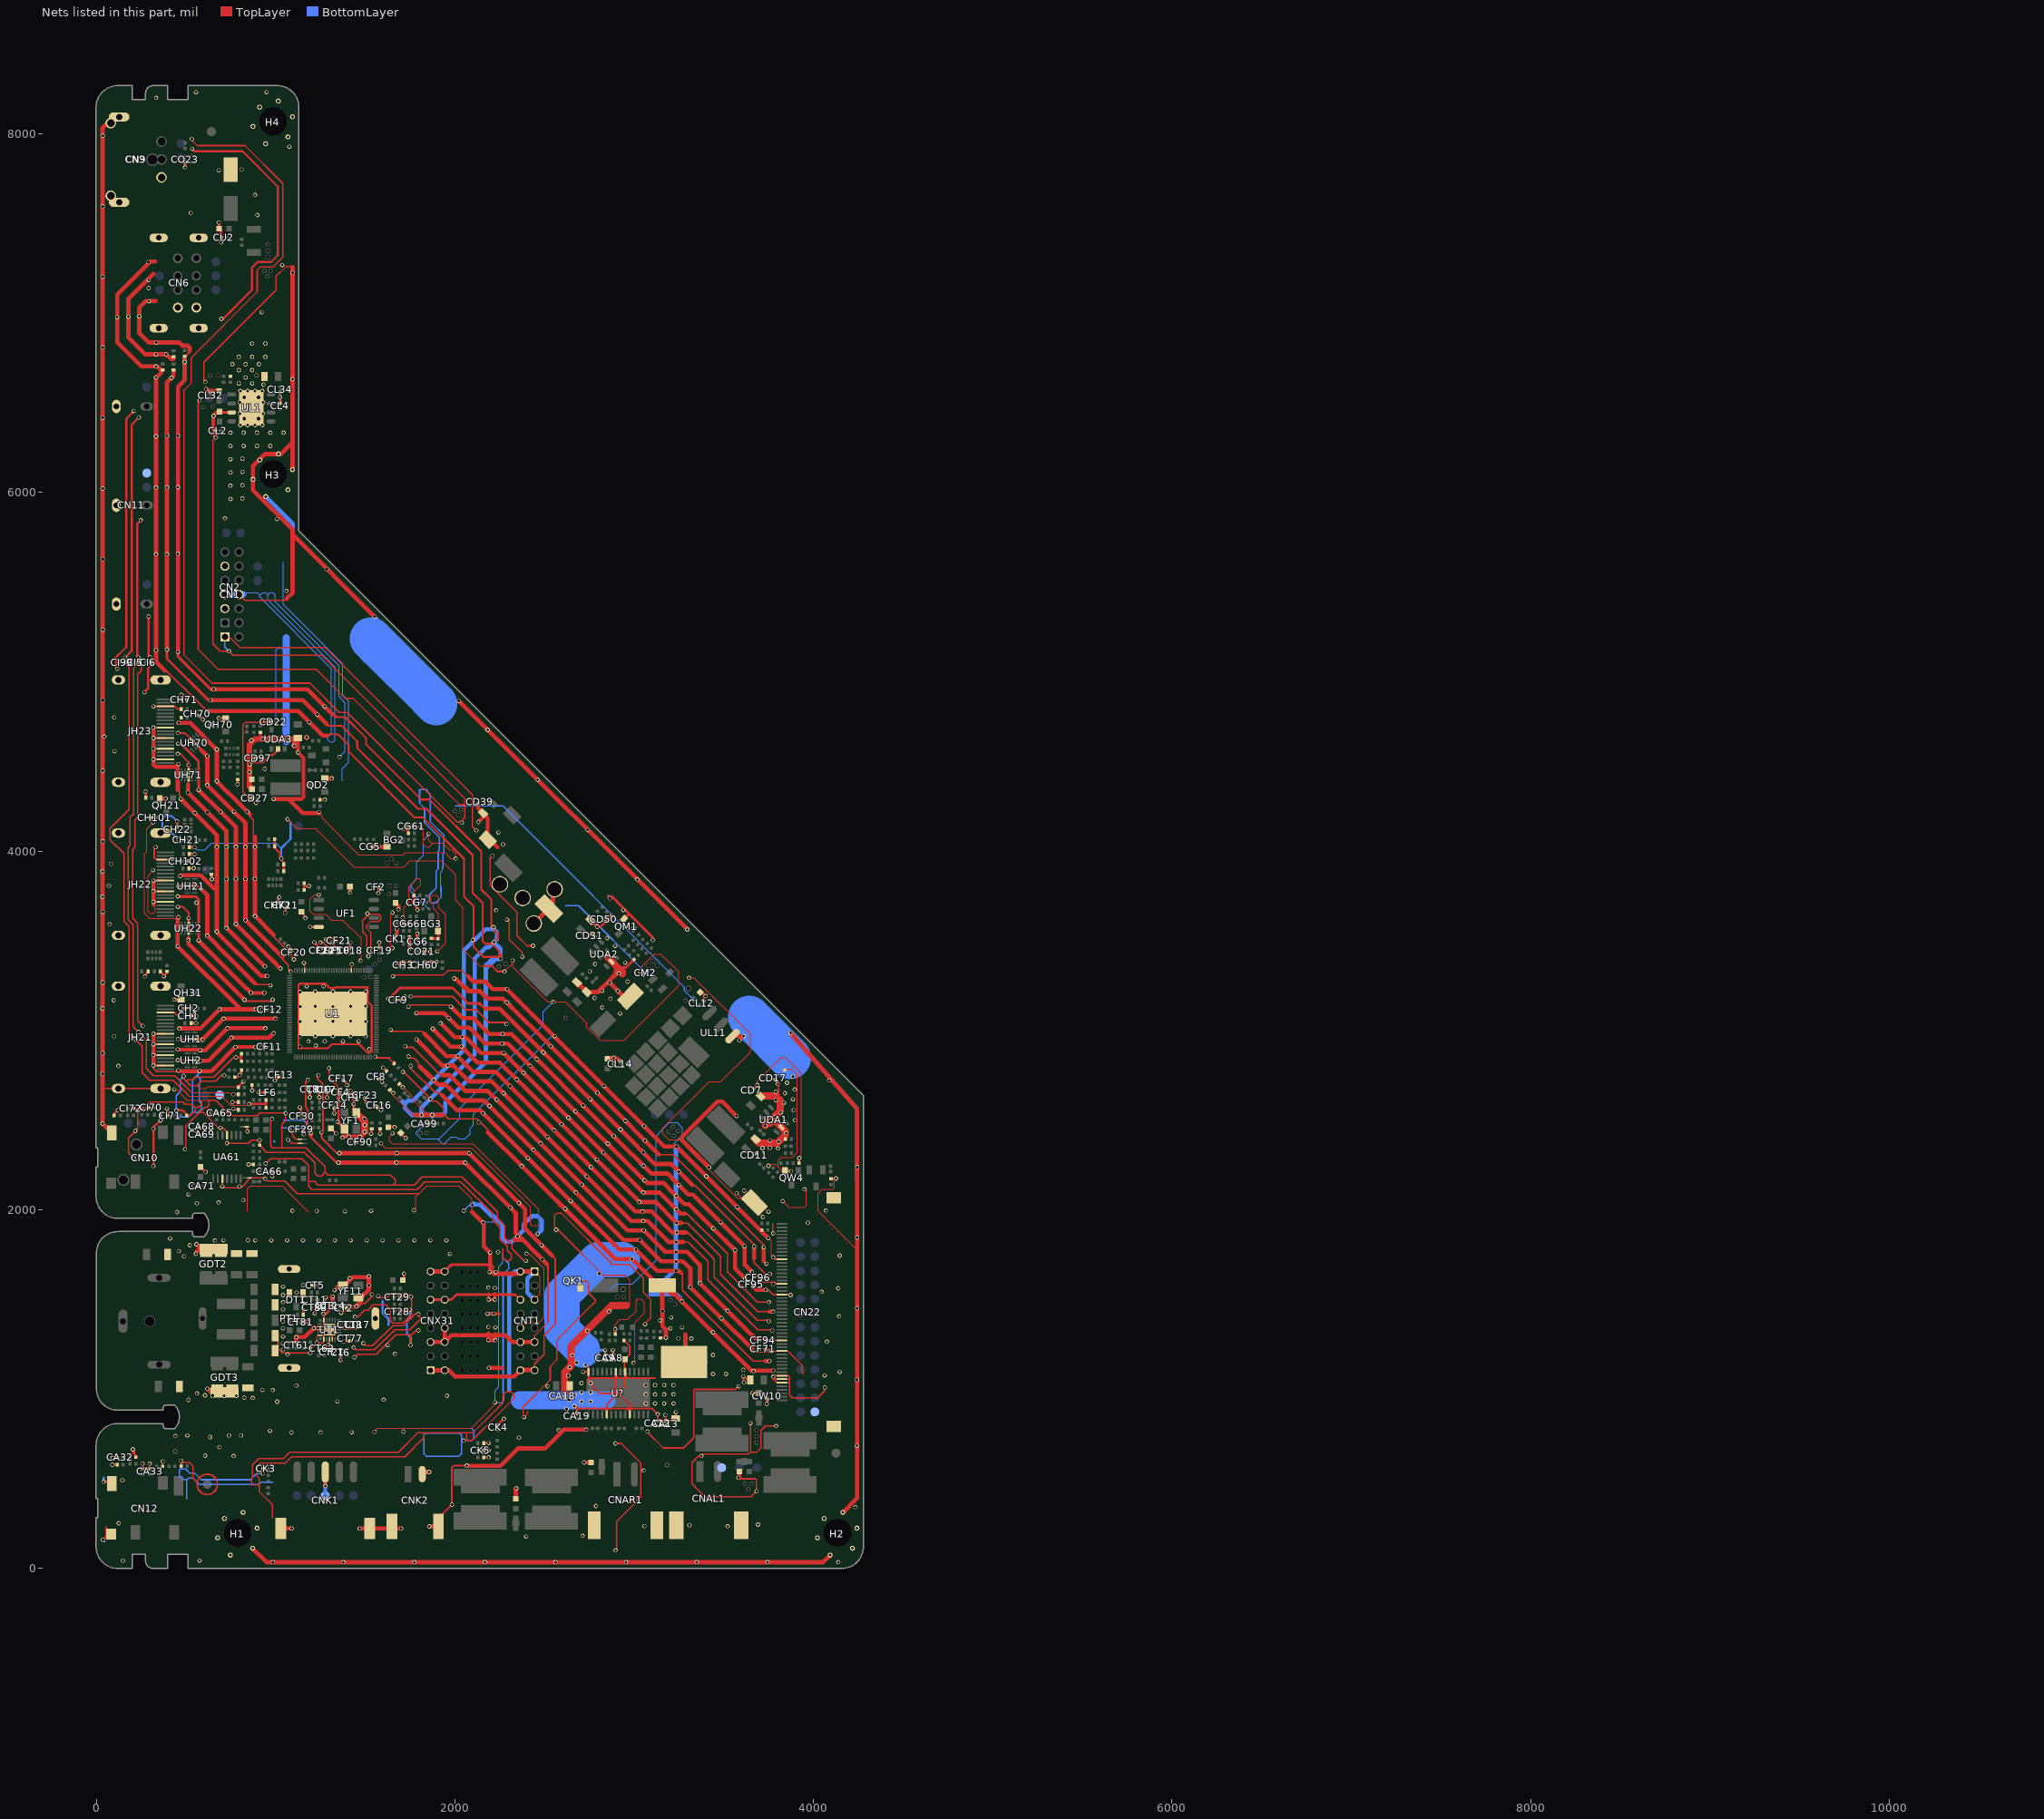
[diagram p0: the nets of this part, all layers, seen from the top]
# Altium PCB MISC105950.PcbDoc (part 7 of 15)
Units mil, origin at the board's own origin, x right, y up, seen from the top; angles counter-clockwise.
Board outline 4280.62 x 8272.76 mil, 2 copper layers (TopLayer, BottomLayer), stack 61.855 mil thick; 541 components, 268 nets, 2324 pads, 1157 vias.

## Via types
v1: diameter 23.62, hole 15.75, TopLayer to BottomLayer, tented both sides, 1087 vias
v2: diameter 23.62, hole 15.75, TopLayer to BottomLayer, 51 vias
v3: diameter 27.56, hole 19.68, TopLayer to BottomLayer, 15 vias
v4: diameter 31.5, hole 19.68, TopLayer to BottomLayer, tented both sides, 4 vias

## Nets (pads, with @x,y where several pads share a name; then routed paths per layer and width w, separated by ;. In a path a pad name is that pad's centre, name@x,y a point inside that pad or via, vN(x,y) a via of type N, cw(c..) or ccw(c..) an arc to the next point about the centre after c; other vN are vias at no path point) (continued)
GND: AV_GND.1 BG2.E BG3.E CA1.1 CA2.1 CA7.1 CA8.1 CA9.1 CA12.1 CA13.1 CA18.1 CA19.1 CA20.1 CA21.2 CA22.1 CA23.2 CA32.2@114.76,617 CA32.2@121.65,617 CA33.2@297,548.35 CA33.2@297,555.24 CA65.2@671.26,2539.5 CA65.2@678.15,2539.5 CA66.1 CA68.2@568.93,2461.69 CA68.2@575.82,2461.69 CA69.2@568.93,2420 CA69.2@575.82,2420 CA70.2 CA71.2@568.61,2131.5 CA71.2@575.5,2131.5 CA99.1 CD7.2@3661.5,2671 CD7.2@3666.37,2675.87 CD11.1 CD17.2@3780.46,2727.54 CD17.2@3785.33,2722.67 CD22.1 CD25.1 CD26.1 CD27.1 CD30.1 CD31.2@2755.96,3534.46 CD31.2@2760.83,3539.33 CD39.2@2126.67,4262.67 CD39.2@2131.54,4267.54 CD50.2@2835.96,3612.04 CD50.2@2840.83,3607.17 CD53.2 CD54.2 CD57.2 CD77.1 CD96.1 CD97.2@884.04,4517.5 CD97.2@890.93,4517.5 CD99.2 CD101.A CD102.A CF1.1 CF2.1 CF3.1 CF4.1 CF5.1 CF6.1 CF7.1 CF8.1 CF9.1 CF10.1 CF11.2@946.54,2907 CF11.2@953.43,2907 CF12.1 CF13.1 CF14.1 CF15.1 CF16.1 CF17.1 CF18.2@1414,3454.35 CF18.2@1414,3461.24 CF19.2@1577,3455.84 CF19.2@1577,3462.73 CF20.1 CF21.2@1335.43,3500.5 CF21.2@1342.32,3500.5 CF23.1 CF24.1 CF25.2@1299.5,3454.18 CF25.2@1299.5,3461.07 CF29.2@1149.35,2447 CF29.2@1156.24,2447 CF30.2@1144.5,2530.07 CF30.2@1144.5,2536.96 CF58.1 CF59.1 CF71.1 CF90.2@1452.26,2377 CF90.2@1459.15,2377 CF94.1 CF95.1 CF96.1 CG5.1 CG6.1 CG7.1 CG61.1 CG66.1 CH1.2@522.35,3081 CH1.2@529.24,3081 CH2.2@495.76,3123 CH2.2@502.65,3123 CH3.1 CH21.2@483.61,4062.1 CH21.2@490.5,4062.1 CH22.2@449.5,4131.35 CH22.2@449.5,4138.24 CH60.1 CH70.2@568.47,4758.03 CH70.2@573.35,4753.15 CH71.2@498.34,4843.5 CH71.2@505.23,4843.5 CH72.1 CH101.1 CH102.1 CI5.1 CI6.1 CI70.1 CI71.1 CI72.1 CI99.1 CK1.1 CK3.2@928.26,554.5 CK3.2@935.15,554.5 CK4.1 CK5.1 CK11.2@1053.5,3681.67 CK11.2@1053.5,3688.56 CL1.1 CL2.1 CL4.2@1023.5,6492.85 CL4.2@1023.5,6499.74 CL10.2 CL11.1 CL12.1 CL13.1 CL14.1 CL31.2 CL32.2@635.43,6553.11 CL32.2@635.43,6560 CL34.1 CM2.1 CN1.1 CN1.5 CN1.7 CN1.8 CN1.11 CN2.3 CN2.5 CN2.6 CN2.9 CN3.2 CN3.3 CN6.4 CN6.8 CN6.9 CN6.10 CN6.11 CN6.12 CN9.3 CN9.4 CN9.5 CN10.2 CN11.2 CN11.4 CN11.6 CN12.1 CN12.2 CN22.6 CN22.7 CN22.8 CN22.15 CN22.18 CN22.31 CN22.34 CN22.41 CN22.52 CN22.53 CNAL1.3 CNAL1.4 CNAR1.3 CNAR1.4 CNK1.3 CNK1.6 CNK1.7 CNK2.2 CNK2.3 CNK2.4 CNT1.1 CNT1.2 CNT1.5 CNT1.6 CNT1.10 CNT1.11 CNT1.12 CNT1.15 CNT1.16 CNX31.1 CNX31.2 CNX31.5 CNX31.6 CNX31.8 CNX31.11 CNX31.12 CNX31.15 CNX31.16 CO21.1 CO23.1 CT2.1 CT3.1 CT5.2@1200.76,1577 CT5.2@1207.65,1577 CT6.1 CT8.1 CT10.2@1241,2652.76 CT10.2@1241,2659.65 CT11.1 CT14.1 CT17.2@1455,1340.76 CT17.2@1455,1347.65 CT18.1 CT21.1 CT28.1 CT29.2@1686.85,1510.5 CT29.2@1693.74,1510.5 CT41.1 CT42.1 CT43.1 CT44.1 CT45.2 CT46.2 CT47.2 CT48.2 CT49.2 CT50.2 CT51.2 CT52.2 CT53.2 CT61.2@1114.5,1252.35 CT61.2@1114.5,1259.24 CT62.2@1266.35,1224.5 CT62.2@1273.24,1224.5 CT77.1 CT80.1 CT81.2@1146.85,1372.5 CT81.2@1153.74,1372.5 CT88.2@1224.83,1453.9 CT88.2@1231.72,1453.9 CU1.1 CU2.2@694.26,7423.88 CU2.2@701.15,7423.88 CW9.1 CW10.1 DA51.A DA52.A DA53.A DH1.A DH2.A DH3.A DH4.A DH21.A DH22.A DH23.A DH70.A DH71.A DH72.A DH73.A DH74.A DH75.A DH76.A DH81.A DI2.A DI3.A DI22.A DI23.A DI24.A DI33.A DI34.A DK2.A DK3.A DK4.A DK70.A DM4.A DO21.A DT1.1 DT1.3 DU1.A DU2.A DU11.A DU12.A DU31.A DU32.A DU33.A DU34.A EA1.2 EA33.2 EA34.2 ED6.2 EU1.2 GDT2.2@613,1754.07 GDT2.2@653,1779.67 GDT2.2@693,1754.07 GDT3.2@674.5,1004.93 GDT3.2@714.5,979.33 GDT3.2@754.5,1004.93 GND_AMP.1 GND_KEY.1 GND_TP.1 H1.1 H1.2 H1.3 H1.4 H1.5 H1.6 H2.1 H2.2 H2.3 H2.4 H2.5 H2.6 H3.1 H3.2 H3.3 H3.4 H3.5 H3.6 H4.1 H4.2 H4.3 H4.4 H4.5 H4.6 HSA1.1 JH21.2 JH21.5 JH21.8 JH21.11 JH21.17 JH21.20 JH21.21 JH21.22 JH21.23 JH22.5 JH22.8 JH22.11 JH22.17 JH22.20 JH22.21 JH22.22 JH22.23 JH23.2 JH23.5 JH23.8 JH23.11 JH23.17 JH23.20 JH23.21 JH23.22 JH23.23 LF6.1 LT2.1 LT4.1 pad.VIA5@747,5964 pad.VIA5@747,6038 pad.VIA5@747,6112 pad.VIA5@747,6186 pad.VIA5@747,6260 pad.VIA5@747,6334 pad.VIA5@757.5,6716 pad.VIA5@793.5,6609 pad.VIA5@793.5,6683 pad.VIA5@793.5,6757 pad.VIA5@813.5,5967 pad.VIA5@813.5,6041 pad.VIA5@813.5,6115 pad.VIA5@813.5,6189 pad.VIA5@821,6260 pad.VIA5@821,6334 pad.VIA5@831.5,6642 pad.VIA5@831.5,6716 pad.VIA5@867.5,6609 pad.VIA5@867.5,6683 pad.VIA5@867.5,6757 pad.VIA5@867.5,6831 pad.VIA5@895,6260 pad.VIA5@895,6334 pad.VIA5@905.5,6716 pad.VIA5@941.5,6757 pad.VIA5@941.5,6831 pad.VIA5@969,6260 pad.VIA5@969,6334 pad.VIA5@1043,6334 pad.VIA5@2250,3814.5 pad.VIA5@2377,3738 pad.VIA5@2439.5,3595.5 pad.VIA5@2555.5,3786.5 pad.VIA5@2622.57,886.29 pad.VIA5@2632.07,1073.5 pad.VIA5@2639.5,1120 pad.VIA5@2654,1186.93 pad.VIA5@2665.57,966.5 pad.VIA5@2665.86,903 pad.VIA5@2679,1145.43 pad.VIA5@2704.98,928.64 pad.VIA5@2704.98,980.07 pad.VIA5@2704.98,1031.51 pad.VIA5@2737.5,1322.93 pad.VIA5@2756.41,928.64 pad.VIA5@2756.41,980.07 pad.VIA5@2756.41,1031.51 pad.VIA5@2860.15,1431.85 pad.VIA5@3064,917.67 pad.VIA5@3064,969.1 pad.VIA5@3064,1020.53 pad.VIA5@3115.43,917.67 pad.VIA5@3115.43,969.1 pad.VIA5@3115.43,1020.53 pad.VIA5@3166.87,917.67 pad.VIA5@3166.87,969.1 pad.VIA5@3166.87,1020.53 pad.VIA5@3201,1337 pad.VIA5@3218.3,917.67 pad.VIA5@3218.3,969.1 pad.VIA5@3218.3,1020.53 pad.VIA5@3318,1280 pad.VIA5@3439,1188.5 pad.VIA5@3439.21,1082.36 pad.VIA5@3511,1082 PT1.2 PT1.3 PT1.4 QD2.E QH21.E QH31.E QH70.E QK1.E QM1.E QW4.E RA1.2 RA4.JP_2K RA5.JP_2K RA9.1 RA11.1 RA55.1 RA56.1 RA64.JP_2K RA65.JP_2K RA69.1 RA71.1 RD28.1 RD35.1 RD47.2 RD53.2 RD54.1 RD88.1 RF5.1 RF12.2 RF13.2 RF19.2 RG8.1 RG9.1 RH2.2 RH75.2 RH82.2 RI14.2 RI16.2 RI21.1 RI23.1 RI25.1 RI36.1 RL32.1 RO22.1 RW11.1 RW14.2 U1.105 U1.124 U1.EPAD U?.6 U?.8 U?.14 U?.19 U?.24 UA61.4 UA61.10 UDA1.2 UDA2.2 UDA3.2 UF1.4 UH1.GND UH2.GND UH21.GND UH22.GND UH70.GND UH71.GND UL1.3 UL1.EPAD UL11.1 UT1.2 UT1.4 UT1.5 UT1.11 UT1.18 UT1.21 UT1.22 UT1.24 UT1.EPAD YF1.2 YF1.4 YF11.2 YF11.4 YPbPr_GND.1 | length 228401.4
  TopLayer w5: 302.82,3624.68 295.33,3624.68 266.69,3653.32 266.69,3982.99 279.5,3995.8 279.5,4124.14 314.86,4159.5 v1(315.5,4159.5) ; 479.91,6818.97 489.41,6809.47 504.93,6809.47 ; DU1.A@491,6759.65 DU1.A@491,6762.82 ; 501.41,2613 504.72,2609.69 659.31,2609.69 ; 511.56,2637.5 511.56,2636.09 515.96,2631.69 696.81,2631.69 747.83,2580.67 842.99,2580.67 v1(851.16,2588.84) ; DH70.A@515.23,3903.1 540.98,3903.1 v1(541.9,3904.02) ; CH102.1@517.07,3943.6 543.63,3943.6 v1@543.73,3943.5 ; 520.44,2662.56 529.31,2653.69 741.31,2653.69 v1@755,2640 ; 560.6,2691.37 576.28,2675.69 607.69,2675.69 618,2686 786.77,2686 RI21.1@790.27,2682.5 ; 842.38,1988.45 842.38,2118.37 855.86,2131.85 1023.65,2131.85 1036.33,2131.85 1181.38,1986.79 ; 864.5,2589 882,2589 ; v1@1240.5,4211.5 1258.52,4193.48 1258.52,4182.98 1462,3979.5 1709.14,3979.5 1719.95,3990.31 ; v1(1550,759.5) 1570.35,779.85 2090.96,779.85 2145.06,833.94 ; DU33.A@1636.33,2668.17 1654,2650.5 1654,2637.4 1770.2,2521.2 ; v1@1641.84,3457 1641.84,3524.5 ; 1641.84,3630.84 1641.84,3604 ; v1(1651.16,3458.36) 1641.84,3467.67 1641.84,3524.5 ; v1(1651.16,3656.01) 1651.16,3654.16 1641.84,3644.84 1641.84,3604 ; CF15.1@1674,3701.5 CF15.1@1674,3718.5 ; v1@1678,3371 1686,3371 1695.23,3380.23 CH3.1@1709.5,3380.23 ; 1706.95,3977.31 1719.95,3990.31 ; CH3.1@1710.5,3381.23 RH82.2@1749.5,3381.23 RH82.2@1749.5,3385.26 ; CG66.1@1712.27,3595 1712.27,3625.23 1715.68,3628.63 1715.68,3684.18 1742.91,3711.41 1742.91,3802.1 1769.6,3828.79 1769.6,3832.6 1783,3846 1798.5,3846 1809.5,3835 1809.5,3812.69 ; v1@1713.03,2680.03 1760.93,2632.13 1760.93,2624.82 1759.83,2623.72 1759.83,2617.83 1846,2531.66 ; v1(1745,3452.5) v1@1745.23,3452.73 ; 1780,1986.79 1780,2071.74 1840.11,2131.85 2020.58,2131.85 2094.93,2057.5 v1(2094.93,2025) 2094.93,1986.79 ; v1@1792,3676.5 1769.77,3698.73 RG9.1@1769.77,3752 1769.77,3772.96 1809.5,3812.69 ; 1797.15,3800.35 1809.5,3812.69 ; v1(1808,4136) 1822.69,4121.31 1822.69,4036.5 1838.69,4020.5 1855,4020.5 1880,4045.5 ; CH60.1@1828.5,3374.34 RH2.2@1861.61,3374.34 ; v1(1852,4095.5) 1852,4061.81 1868.31,4045.5 1880,4045.5 ; RH2.2@1868.5,3381.23 1896.27,3381.23 v1(1896.5,3381) ; 2152.56,841.44 2145.06,833.94 ; v1(2222.61,924.66) 2226.82,920.44 2231.56,920.44 2145.06,833.94 ; v1(2275,3328) 2321.5,3374.5 v1(2321.5,3389) 2321.5,3353.5 2517,3158 v1(2548,3158) ; 2607.59,3158 v1(2548,3158) ; HSA1.1@3193.65,1175.35 3355.65,1175.35 HSA1.1@3383,1148 ; 3249,3324.61 3249,3250 2941.38,2942.39 2810.11,2942.39 2734.39,3018.11 2734.39,3040.42 2616.81,3158 v1(2548,3158) ; 3653.11,1214.27 3663.24,1204.14 3761.94,1204.14 v1@3768.62,1210.82 ; v1(3746.74,1840.63) 3765.5,1821.87 3765.5,1743.65 v1@3775.92,1733.23 ; 1641.84,3524.5 1641.84,3604 ; 1719.95,3990.31 1944.19,3990.31 1976.5,3958 v1(2004,3958) 2004,3985.81 1984,4005.81 1970.19,4005.81 1930.5,4045.5 1880,4045.5
  TopLayer w6: 302.82,3624.68 v1@448.84,3624.68 ; v1(314.5,3893.5) 314.5,3890.35 287.19,3863.04 287.19,3661.81 297,3652 315.02,3652 ; 315.21,3652.19 326.81,3663.79 326.81,3671.81 326.94,3671.94 326.94,3706.8 ; 1078.88,4163.62 v1(1065,4177.5) 1116.5,4126 1222,4126 1436.5,3911.5 1625.5,3911.5 ; 1191.97,3731.62 1191.97,3718 ; 1229,1281.53 1229,1293 1234.5,1298.5 UT1.EPAD@1268,1298.5 ; v1(1240.5,3756.5) 1215,3756.5 1191.97,3733.47 1191.97,3718 ; v1@1470.98,3387.23 1470.98,3400.76 1475.81,3405.6 1475.81,3512.77 1373.15,3615.43 1309.94,3615.43 1279.06,3646.31 1209.81,3646.31 1191.97,3664.15 1191.97,3718 ; v1@1585.63,2364.63 v1@1585.63,2374.19 ; v1(1586,2369) 1610.5,2344.5 2091.48,2344.5 2421,2014.98 2421,1918.31 2427,1912.31 2465.31,1912.31 2465.5,1912.5 ; 1637.5,3911.5 1625.5,3911.5 ; v1(1650.76,2425.26) 1633.81,2408.32 1633.81,2380.69 1649,2365.5 2100.17,2365.5 2465.5,2000.17 2465.5,1892.5 ; DO21.A@1867.5,3512.23 1904,3512.23 v1@1904,3594.5 ; v1@1900.5,3440.5 1946.5,3486.5 1946.5,3644.97 1906,3685.47 1906,3740.5 1894.19,3752.31 1870.31,3752.31 1863.5,3745.5 1863.5,3715 1878,3700.5 1878,3679 1907,3650 1907,3514.23 RO22.1@1904.5,3511.73 ; 2188,3358.5 2137,3358.5 2043.81,3451.69 2043.81,3683.6 2002,3725.41 2002,3867.97 1925.16,3944.81 1747.31,3944.81 1714,3911.5 1625.5,3911.5 ; CNT1.10@2364.47,1339.15 2394.12,1368.8 2467.8,1368.8 2496,1397 2496,1670.08 2412.58,1753.5 v1(2398,1753.5) ; CNT1.2@2364.47,1654.11 CNT1.1@2443.21,1654.11 2475,1622.32 2475,1528.42 CNT1.5@2443.21,1496.63 ; CNT1.11@2443.21,1260.41 2443.21,1297.21 2519,1373 2519,1374.42 ; v1(2460,1863.5) 2465.5,1869 2465.5,1892.5 ; 2465.5,1884.38 2465.5,1892.5 ; v1@2893.67,1333.33 2893.67,1359.67 2920,1386 2963.26,1386 3009.5,1432.24 3009.5,1492 3018.5,1501 3037.33,1501 ; 2950.08,1632 2974.5,1607.58 2974.5,1466.5 ; v1(2995.99,1143.72) 3003.63,1151.36 3003.63,1319.5 ; 3003.63,1348.42 3003.63,1319.5 ; 3010,1489.5 3021.5,1501 3037.33,1501 ; v1(3031,3329) 3043.59,3341.59 3043.59,3356.41 3112.69,3425.5 3148.11,3425.5 3249,3324.61 ; CM2.1@3051.67,3310.17 CM2.1@3051.67,3315.83 ; v1(3054.46,2465.14) 3064.55,2455.05 3069.55,2455.05 ; v1@3059.83,2464.77 3069.55,2455.05 ; 3164.1,2360.5 3069.55,2455.05 ; 3276.46,2375.96 3263.93,2388.5 ; 3287.1,2352.6 3575.7,2064 ED6.2@3646,2064 ; v1(3305.5,3292.5) 3316.5,3292.5 3317,3293 3332,3293 3647,2978 3647,2878.56 3481.44,2713 3417.87,2713 3158.08,2453.21 3158.08,2423.74 3193.32,2388.5 3237.62,2388.5 ; v1(3572,2091) 3623.56,2039.44 ED6.2@3670.56,2039.44 ; v1(3613,2105) 3670.56,2047.44 ED6.2@3670.56,2039.44 ; CD99.2@3677.11,2392.67 3677.11,2377.39 3698,2356.5 ; v1@3690.53,2700.03 v1(3685.5,2695) 3685.5,2715.95 3816.55,2847 3843.53,2847 3931.1,2759.43 3931.1,2313.5 ; v1(3717,1958) 3670.56,2004.44 ED6.2@3670.56,2039.44 ; v1(3748,1987.5) 3696.06,2039.44 ED6.2@3670.56,2039.44 ; v1(3748,2244) 3756.56,2252.56 3785.44,2252.56 3801.68,2236.32 ; 3777.5,2493.46 UDA1.2@3804.98,2465.98 ; v1(3827.64,2046.86) 3863,2011.5 3948,2011.5 3958.5,2022 3958.5,2072.5 ; 3835.86,2435.1 UDA1.2@3804.98,2465.98 ; RD28.1@3838.98,2778.52 3844.98,2784.52 3876.32,2784.52 3910.1,2750.73 3910.1,2319.06 3882.04,2291 3819.52,2291 3801.68,2273.15 3801.68,2236.32 ; QW4.E@3840.5,2216 3822,2216 3801.68,2236.32 ; 3853.5,2390.5 3853.5,2417.46 UDA1.2@3804.98,2465.98 ; v1@3919.5,2286 3931.1,2297.6 3931.1,2313.5 ; 3931.1,2297.5 3931.1,2313.5 ; v1(3949,2113) 3958.5,2103.5 3958.5,2072.5 ; 3958.5,2081.5 3958.5,2072.5 ; 4112.77,2121.27 4106.14,2114.64 ; 4115.34,2127.07 4115.34,2154.01 ; v1(4125.15,2172.73) RW11.1@4097.5,2172.73 4097.5,2171.86 4115.34,2154.01 ; 4243.09,1784 4232.17,1784 4024.5,1991.67 4024.5,2091 4048.14,2114.64 4106.14,2114.64 ; 3003.63,1319.5 3003.63,1370.68 3055.45,1422.5 3055.45,1482.87 3037.33,1501 ; 3237.62,2388.5 3263.93,2388.5 ; 3237.62,2388.5 3242.03,2392.91 3245.34,2392.91 3247.23,2391.02 3266.45,2391.02 3263.93,2388.5 ; 4106.14,2114.64 4115.34,2123.84 4115.34,2154.01
  TopLayer w7: CI99.1@155.01,5050.33 181.31,5024.03 181.31,5008.84 ; 179.47,4229 75.5,4125.03 75.5,4063.5 152.5,3986.5 152.5,3605.87 180.5,3577.87 180.5,2985.5 v1(219,2947) 254,2912 254,2764.5 297.21,2721.29 427.77,2721.29 511.56,2637.5 ; 181.31,4229 181.31,5008.84 ; 181.31,5011.69 181.31,5008.84 ; 205.31,4206.5 187,4188.19 187,4029.03 176.5,4018.53 176.5,3615.81 204.5,3587.81 204.5,3020 278,2946.5 278,2785.5 318.21,2745.29 437.71,2745.29 520.44,2662.56 ; 205.31,4207 205.31,5021.03 233.73,5049.45 CI5.1@233.73,5052 250.5,5035.23 250.5,5006 229.31,4984.81 229.31,4189.81 214,4174.5 214,4020.81 200.5,4007.31 200.5,3625.75 228.5,3597.75 228.5,3053.5 v1(257.5,3024.5) ; CI72.1@207.23,2564 229,2564 ; v1(207.5,2286.5) 177.5,2316.5 177.5,2400 v1(216,2438.5) 229,2451.5 229,2564 ; CI70.1@283.77,2564 229,2564 ; CI70.1@288.27,2568.5 288.27,2591.27 295.5,2598.5 481.22,2598.5 493.03,2586.69 532.59,2586.69 550.09,2569.19 ; v1(317,2803) 317,2787.27 334.42,2769.85 v1@448.34,2769.85 ; v2@446.67,1983.5 v2(448.81,1985.65) ; 461.61,4383.82 461.61,4311.02 510.05,4262.58 510.05,4250.55 ; v1@486,2743 486,2730.94 525.57,2691.37 560.6,2691.37 584.6,2715.37 664.09,2715.37 697.72,2749 v1(711.6,2749) ; v1(492.75,2336.25) 498,2341.5 498,2465.53 602.16,2569.69 613.91,2569.69 625.81,2581.59 625.81,2608.5 626,2608.69 ; 501.97,2714.97 509.69,2722.69 534.41,2722.69 551.1,2739.37 654.15,2739.37 ; DI24.A@502.46,2524.5 523.03,2524.5 550.09,2551.56 550.09,2569.19 ; 585,2608.69 585,2587.28 566.91,2569.19 550.09,2569.19 ; 611.5,2739.37 654.15,2739.37 ; 617,2608.69 663.99,2608.69 748.68,2524 781.5,2524 ; v1(691,2456) v1@693.5,2453.5 ; v1(701.5,2129.5) 701.59,2129.59 UA61.10@701.59,2171.5 701.59,2133.87 715.5,2119.96 804.37,2119.96 815.46,2131.04 ; 723.5,2549.18 723.5,2541.36 740.86,2524 781.5,2524 ; v1(727.18,2370.82) 729,2369 846,2369 864,2387 v1(909,2387) ; v1(763,2642.5) DI22.A@789.77,2642.5 ; v1(778.54,2848.54) 763.31,2848.54 654.15,2739.37 ; v1(797.5,2128.5) 812.91,2128.5 815.46,2131.04 ; 854.96,4205.46 854.96,4193.44 875,4173.4 875,4101.5 ; RA65.JP_2K@857.75,2173.34 815.46,2131.04 ; RA65.JP_2K@860.41,2176 932,2176 v1@941,2167 ; v1(868.16,2664.16) v1@870.5,2666.5 ; 875,4050 875,4101.5 ; 875,4085 875,4101.5 ; 876.73,3268.5 891.41,3253.81 966.85,3253.81 v1(970.35,3250.31) ; RA69.1@909.23,2359.25 949.14,2319.34 1158.78,2319.34 1218.11,2260.02 1218.11,2203.12 1233.72,2187.5 1253.5,2187.5 1274.5,2208.5 ; v1(941,2171) 952.15,2159.85 1047.92,2159.85 1071.58,2136.19 ; v1(943,2256.5) 970.84,2284.34 1144.29,2284.34 1183.11,2245.52 1183.11,2130.89 1201.81,2112.19 1787.93,2112.19 1830.58,2154.85 2031.52,2154.85 2209.84,1976.53 2209.84,1941.31 2251.69,1899.46 2251.69,1833.46 2291.19,1793.96 2291.19,1772.23 2314.5,1748.92 2314.5,1725.28 2302.41,1713.19 2285.59,1713.19 2266.19,1732.59 2266.19,1781 ; 962.24,3545.74 1086.21,3421.76 1086.21,3409.47 v1@1102.38,3393.3 ; 978.34,3403.77 1032.5,3349.61 1027.26,3344.37 v1(1025.69,3344.37) ; v1(978.5,2505) 972.5,2505 969.5,2502 969.5,2356.84 982,2344.34 1169.14,2344.34 ; 1035,2344.34 1035,2475.47 1054.66,2495.13 v1(1054.66,2537.66) 910.25,2537.66 896.59,2524 781.5,2524 ; 1036.74,3408.3 1036.74,3396.28 1070,3363.02 1070,3340.38 v1(1082.78,3327.6) ; 1059.08,2148.7 1071.58,2136.19 ; v1@1076.5,2389.5 v1(1068,2389.5) 1089.16,2368.34 RA4.JP_2K@1136.8,2368.34 ; v1(1092.5,2450) 1095,2447.5 1095,2408.78 1111.43,2392.34 RA5.JP_2K@1134.8,2392.34 RA5.JP_2K@1133.66,2392.34 ; 1118.74,2344.34 1169.14,2344.34 ; 1187.42,2155.81 1215.91,2155.81 1234.53,2137.19 1772.18,2137.19 1816.99,2182 2039.72,2182 2215.31,2006.41 ; v1(1216.5,1420.5) v1@1218,1422 ; v1@1220.42,1330 UT1.22@1246.35,1330 UT1.EPAD@1299.5,1330 ; v1@1221.1,1345.75 UT1.21@1246.35,1345.75 UT1.EPAD@1283.75,1345.75 ; RD47.2@1247.23,4287 v1(1274,4287) ; 1260.78,1256.5 1268,1263.72 UT1.2@1268,1276.85 1268,1298.5 UT1.EPAD@1299.5,1330 ; v1(1265.5,1419.5) 1265.62,1419.62 1283.38,1419.62 ; CT3.1@1278.5,1484.91 v1(1278.5,1509) ; UT1.EPAD@1280.8,1345.75 1268.63,1357.92 1268.63,1382.52 UT1.18@1268,1383.15 1268,1404.24 1283.38,1419.62 ; 1294.34,1469.07 1294.34,1430.58 1283.38,1419.62 ; v2@1295.48,1246 v2(1294.25,1244.78) 1299.5,1250.02 UT1.4@1299.5,1276.85 ; v1(1296.85,2788.14) 1296.85,2737.07 1342.81,2691.11 1342.81,2614.19 1347.5,2609.5 ; UT1.5@1315.25,1277.85 UT1.EPAD@1315.25,1315.25 ; v1@1315.5,1504.97 1315.5,1499 1317.5,1497 CT14.1@1317.5,1472.23 ; v1@1347.5,2486 1347.5,2522.5 ; v1@1347.5,2487.27 YF1.4@1382.57,2452.2 ; v1@1360,1422.11 1370.39,1432.5 1380.5,1432.5 ; v1(1361,1160) 1361,1186.27 CT6.1@1361.5,1186.77 ; v1(1364.5,1423) 1371,1423 1380.5,1432.5 ; YF1.4@1382.57,2471.89 YF1.4@1382.57,2476.93 ; v1(1384.5,1338.5) v1@1386.77,1340.77 ; v1@1387,1337 1381.5,1337 1372.75,1345.75 UT1.11@1352.65,1345.75 1315.25,1345.75 UT1.EPAD@1299.5,1330 ; CT2.1@1393.23,1450 1406.23,1463 1441.5,1463 YF11.4@1470.31,1491.81 ; v1@1444,1408 1442,1406 v1(1442,1402) 1458.24,1402 1493.85,1437.61 1513.67,1437.61 1543.56,1467.5 1563,1467.5 ; 1446,1218.5 v1(1434.5,1230) 1448,1216.5 1550.97,1216.5 1662.97,1328.5 1747.47,1328.5 1805.97,1387 1805.97,1398.53 v1@1787.53,1416.97 ; CT17.2@1451.24,1337 CT17.2@1455,1340.76 ; 1455.5,1192 v1(1439,1175.5) 1456,1192.5 1560.91,1192.5 1624.21,1255.79 ; v1(1487.5,1254) 1501,1240.5 1541.03,1240.5 1653.03,1352.5 1713,1352.5 1777.47,1416.97 v1@1787.53,1416.97 ; v1(1535.5,1526.5) 1535.5,1513.18 1497.93,1475.61 1478.11,1475.61 1454,1451.5 1425.5,1451.5 1406.5,1432.5 1380.5,1432.5 ; v1(1570.5,1517) 1579,1508.5 1619.57,1508.5 1639.91,1528.84 1668,1528.84 ; 1589.82,1467.5 1563,1467.5 ; v1(1624,1243.5) 1624.21,1243.71 1624.21,1255.79 ; v1(1640.5,3002.5) 1649,2994 1814.7,2994 1828.35,2980.35 ; 1642.91,1528.84 1668,1528.84 ; 1654.91,2137.19 1666.81,2149.09 1666.81,2165.91 1639.72,2193 1290,2193 1274.5,2208.5 ; v1(1709.37,2768) 1711.53,2768 1873.55,2605.98 1873.55,2603.81 1897.89,2603.81 1937.17,2564.53 1937.17,2532.98 ; 1725.5,1383 1710.5,1368 ; v1(1740,2853.5) 1748.69,2844.81 1770.85,2844.81 1796.81,2818.85 1796.81,2794.4 1894.53,2696.68 1906.55,2696.68 ; v1(1740.26,3131.27) v1@1745.49,3136.5 ; v1@1745.49,3141 v1@1972.02,3141 ; v1(1751.25,1243.02) 1749.5,1244.77 1749.5,1301 ; v1(1752.5,2800.5) 1752.5,2787.8 1888.12,2652.18 1912.46,2652.18 1924.32,2640.32 ; v1@1779.22,3095.81 1781.53,3093.5 1940.06,3093.5 1955.3,3078.27 1949.69,3083.87 ; v1(1795.47,1416.97) v1@1787.53,1416.97 ; v1(1795.5,1325.5) 1783.36,1325.5 1758.86,1301 1749.5,1301 ; 1798.51,2088.19 1119.58,2088.19 1071.58,2136.19 ; 1931.5,2527.31 1937.17,2532.98 ; v1(2132.48,2485.8) 2142.93,2485.8 2152.11,2476.61 ; v1@2160.66,1921.07 v1@2160.66,1925.93 ; 2183.46,2430.71 2183.46,2445.27 2152.11,2476.61 ; v1(2192.5,1651) 2197.5,1656 v1@2228,1656 ; 2217,2004.72 2215.31,2006.41 ; v1(2395,1714.5) 2393.5,1716 2382.78,1716 2316.19,1782.59 2316.19,1804.31 2276.69,1843.81 2276.69,1909.81 2234.84,1951.66 2234.84,1986.89 2215.31,2006.41 ; CNT1.15@2443.21,1102.93 2443.21,1139.02 2497.36,1193.18 2497.36,1299.75 2558,1360.38 2558,1374.5 ; CNT1.11@2443.21,1260.41 2443.21,1296.51 ; 2737.5,1875.41 2740.71,1872.21 ; 3137.38,2307 3217.44,2307 3722,1802.44 3722,1778 ; 3213.99,1871.55 3299.34,1871.55 3445.95,1724.94 3445.95,1622.43 3686.01,1382.38 3745,1382.38 v1(3750.5,1376.88) ; 3252.5,1818.55 3301.43,1818.55 3409.95,1710.02 3409.95,1607.52 3687.6,1329.88 3763.5,1329.88 v1(3769.5,1323.88) ; 3262,1924.55 3297.25,1924.55 3481.95,1739.85 3481.95,1637.34 3689.27,1430.03 v1@3774.85,1430.03 ; 3267.95,1647.69 3267.95,1548.7 3662.22,1154.44 3730,1154.44 ; 3279.85,2030.55 3293.08,2030.55 3562.45,1761.17 ; 3281.5,1977.55 3295.17,1977.55 3517.95,1754.76 3517.95,1652.25 3687.18,1483.03 v1(3751.25,1483.03) ; 3323.76,2136.55 3336.98,2136.55 3668.45,1805.08 v1@3668.45,1791.5 ; v1@3553.95,1769.67 3562.45,1761.17 ; 3562.45,1732 3562.45,1761.17 ; 3649.04,1317.52 3677.95,1288.61 3719.5,1288.61 ; 3668.45,1725.88 3668.45,1702.57 3730.71,1640.32 v1(3755.86,1640.32) v1@3750.92,1635.38 ; CF96.1@3703.59,1604.51 3712.09,1596.01 3738.5,1596.01 ; 3721.5,1742.88 3721.5,1712.19 v1(3737.41,1696.28) ; 3722,1711.69 v1(3737.41,1696.28) ; 3724.11,1596.01 3738.5,1596.01 ; 3728.27,1288.61 3719.5,1288.61 ; CF94.1@3733.24,1270.18 3758.7,1270.18 v1(3760,1268.88) ; v1(3733.68,1551.51) 3745.71,1551.51 3771.44,1525.78 CN22.31@3823.43,1525.78 3869.22,1525.78 v1(3872,1523) ; 3741.47,1429.88 v1(3775,1429.88) ; v1@3743,1702.45 3743,1701.88 v1(3737.41,1696.28) ; 3747.01,1269.87 v1@3760.5,1269.87 ; v1(3775,1584.88) 3775.05,1584.83 CN22.34@3823.43,1584.83 3794.18,1584.83 3783,1596.01 3738.5,1596.01 ; v1(3775.11,1067.56) v1@3775.11,1070.11 ; CN22.18@3823.43,1269.87 v1@3760.5,1269.87 ; CN22.7@3853.16,1053.34 CN22.7@3823.43,1053.34 ; 3864.35,1033.65 CN22.6@3823.43,1033.65 3797.23,1033.65 3775.11,1055.77 v1@3775.11,1070.11 ; 3864.66,1053.34 CN22.7@3823.43,1053.34 ; 3865,1025.5 3865,1018.5 ; v1@3871.72,1525.78 3871.72,1523.28 v1(3872,1523) ; v1@3878.17,1523 v1(3872,1523) ; 4064.5,990 4023,948.5 3882.28,948.5 3865,965.78 3865,1018.5 ; 1169.14,2344.34 1274.5,2238.98 1274.5,2208.5 ; 1563,1467.5 1612.41,1467.5 1640,1439.91 1640,1380.5 1652.5,1368 1710.5,1368 ; 1624.21,1255.79 1669.41,1301 1749.5,1301 ; 1668,1528.84 1743.16,1528.84 1757.5,1514.5 1757.5,1415 1710.5,1368 ; 1937.17,2532.98 1963.3,2506.84 2121.88,2506.84 2152.11,2476.61 ; 3719.5,1288.61 3730.27,1288.61 3734.73,1284.15 3734.73,1270.18 3735.03,1269.87 v1@3760.5,1269.87 ; v1@3775.11,1070.11 3791.88,1053.34 CN22.7@3823.43,1053.34 ; v1@3775.11,1070.11 3778.02,1073.02 CN22.8@3823.43,1073.02 3857.48,1073.02 3865,1065.5 3865,1018.5